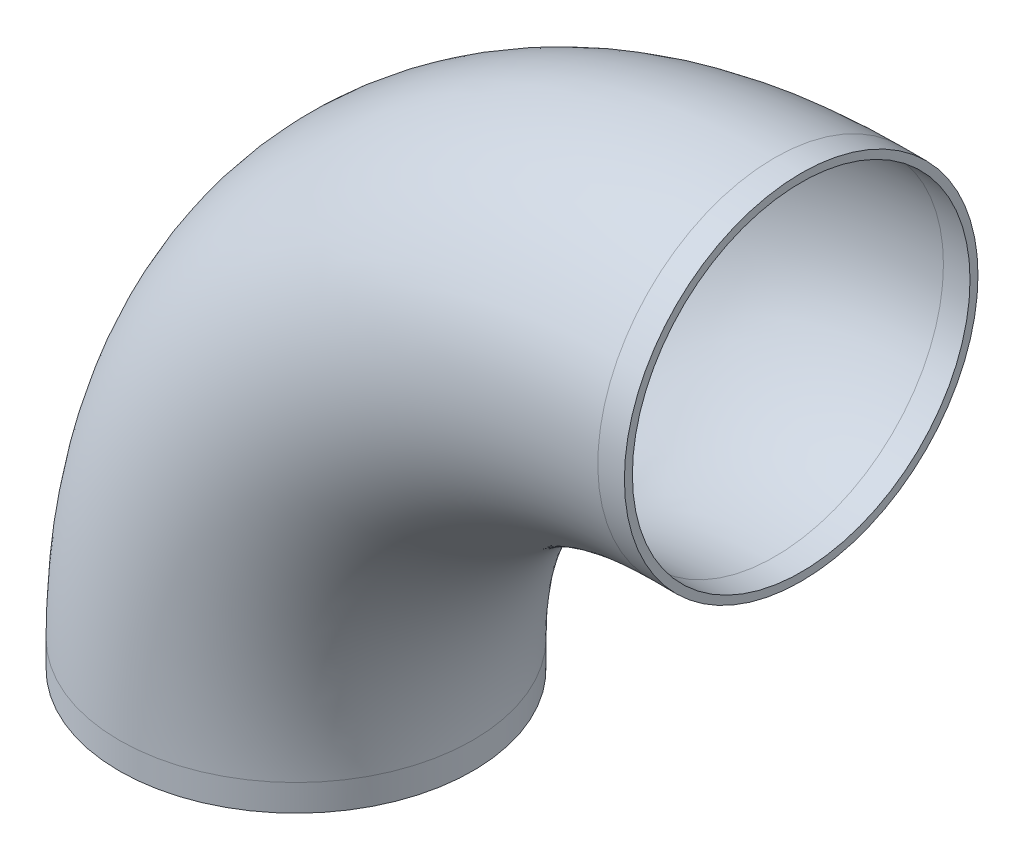
from build123d import *

# Parameters (mm, degrees)
SKETCH1_R = 66.5
SHELL1_T  = -3


with BuildPart() as part:
    # Sweep1: sweep along a path in Sketch2
    with BuildLine(Plane.XY) as sweep1_path:
        Line((0, 0), (0, 10))
        ThreePointArc((0, 10), (52.720779386, 137.279220614), (180, 190))
        Line((180, 190), (190, 190))
    # Sketch1 → Sweep1 (sweep)
    with BuildSketch(Plane(origin=(0, 0, 0), x_dir=(1, 0, 0), z_dir=(0, 1, 0))):
        Circle(SKETCH1_R)
    sweep(path=sweep1_path.line)

    # Shell1
    shell1_openings = [part.faces().sort_by_distance(p)[0] for p in [
        (190, 190, 0),
        (0, 0, 0),
    ]]
    offset(amount=SHELL1_T, openings=shell1_openings, kind=Kind.INTERSECTION)


solid = part.part
